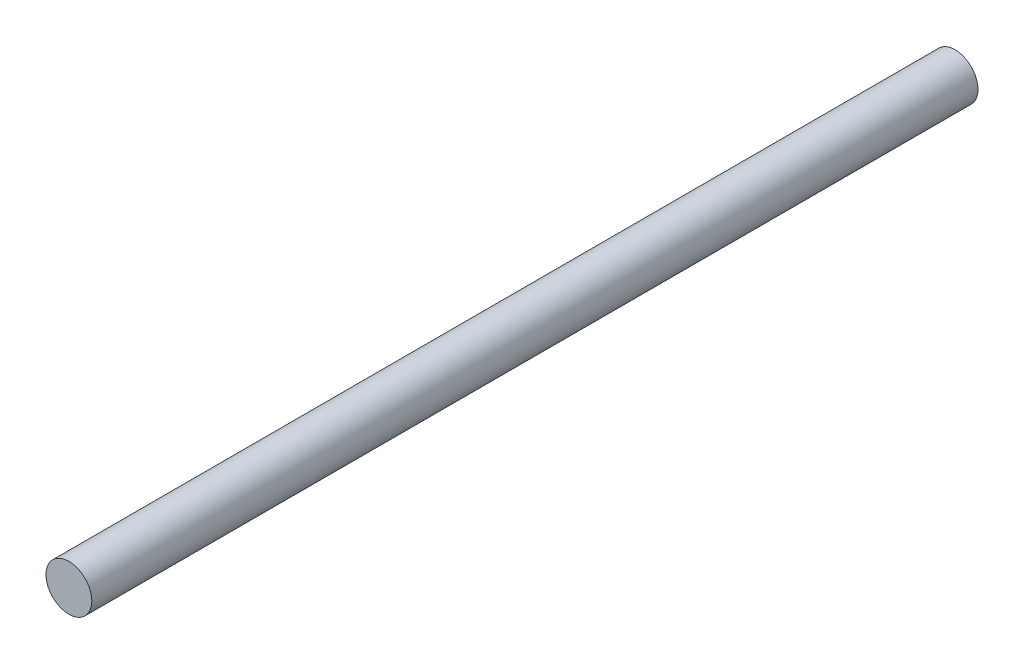
from build123d import *

# Parameters (mm, degrees)
SKETCH1_R           = 4.5
BOSS_EXTRUDE1_DEPTH = 174


with BuildPart() as part:
    # Sketch1 → Boss-Extrude1 (new body)
    with BuildSketch(Plane.XY):
        Circle(SKETCH1_R)
    extrude(amount=BOSS_EXTRUDE1_DEPTH)


solid = part.part
